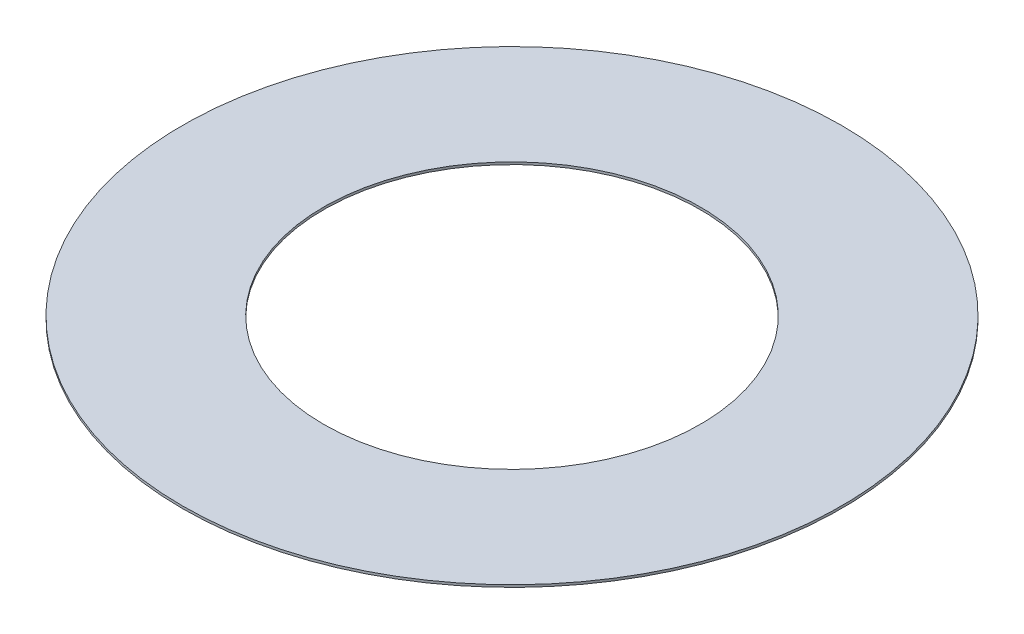
SolidWorks part; units mm, degrees
ref_plane "Front Plane" through (0, 0, 0) normal (0, 0, 1) x (1, 0, 0)
ref_plane "Top Plane" through (0, 0, 0) normal (0, 1, 0) x (1, 0, 0)
ref_plane "Right Plane" through (0, 0, 0) normal (1, 0, 0) x (0, 0, -1)
sketch "Sketch1" plane through (0, 0, 0) normal (0, 1, 0) x (1, 0, 0)
  circle A0 centre (0, 0) radius 7
  circle A1 centre (0, 0) radius 4
  dimension "D1" = 8
  dimension "D2" = 14
extrude "Boss-Extrude1" add sketch "Sketch1" along normal blind 0.05
